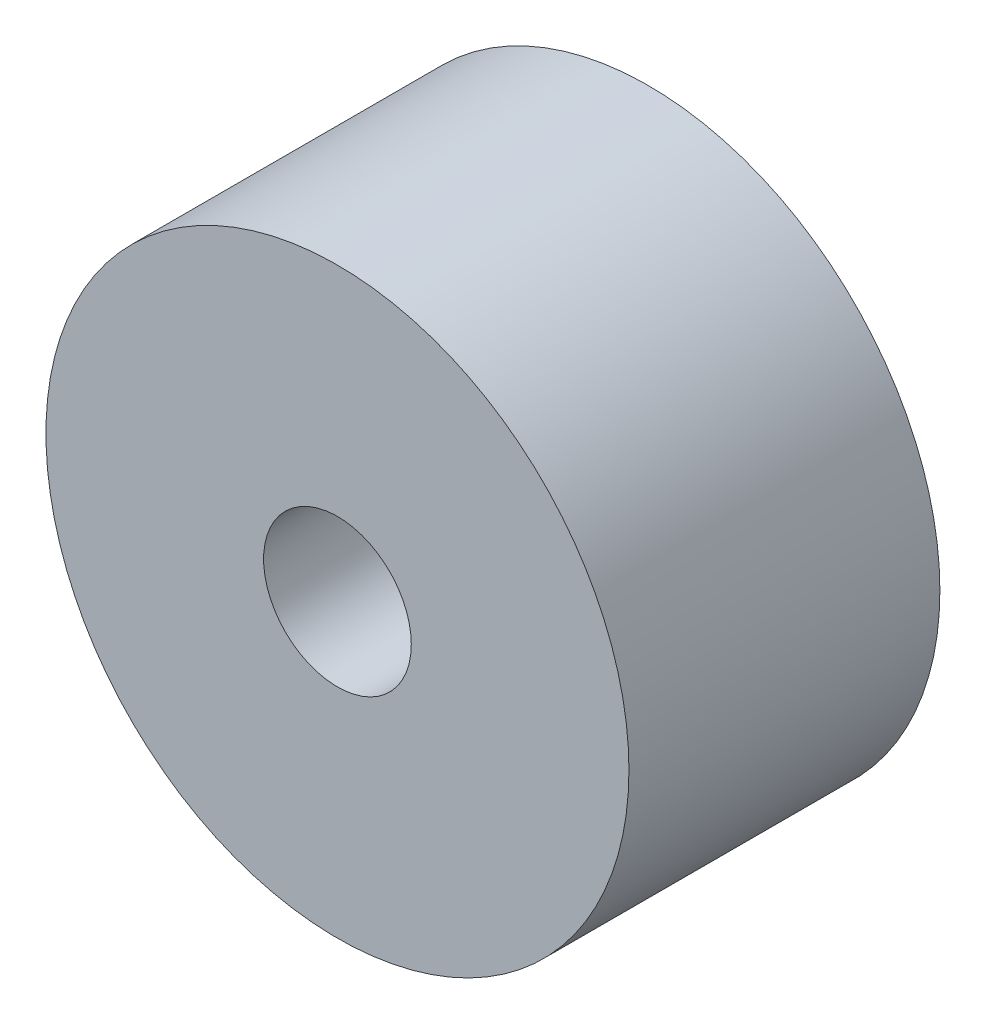
from build123d import *

# Parameters (mm, degrees)
SKETCH_1_R      = 150
SKETCH_1_R_2    = 38
EXTRUDE_1_DEPTH = 80


with BuildPart() as part:
    # 草图1 → 凸台-拉伸1 (new, symmetric)
    with BuildSketch(Plane.XY):
        Circle(SKETCH_1_R)
        Circle(SKETCH_1_R_2, mode=Mode.SUBTRACT)
    extrude(amount=EXTRUDE_1_DEPTH, both=True)


solid = part.part
